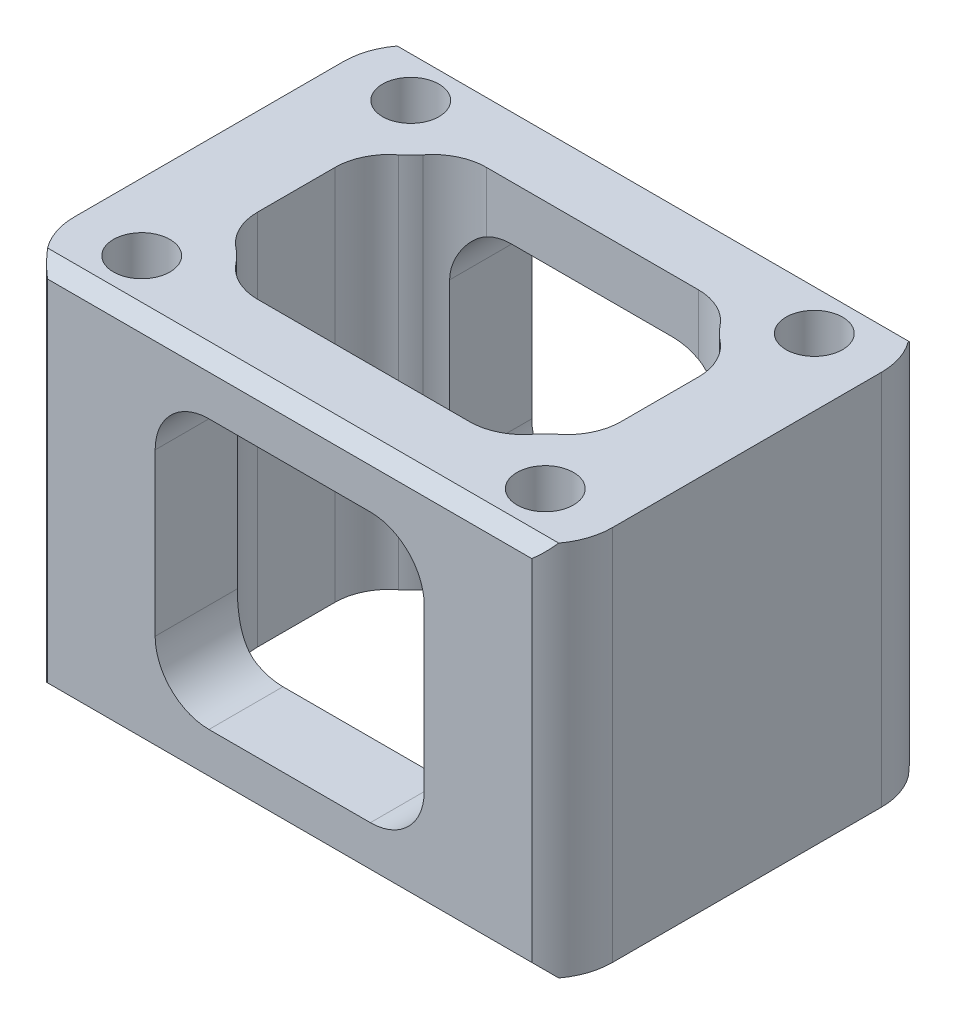
from build123d import *

# Parameters (mm, degrees)
SKETCH_1_W          = 40
SKETCH_1_H          = 28
EXTRUDE_1_DEPTH     = 28
SKETCH_2_R          = 2.1
CUT_EXTRUDE_1_DEPTH = 38.148351242
SKETCH_3_OUTSIDE_W  = 53.256
SKETCH_3_OUTSIDE_H  = 41.256
CUT_EXTRUDE_2_DEPTH = 38.148351242
FILLET_3_R          = 4
SKETCH_6_W          = 20
SKETCH_6_H          = 20
CUT_EXTRUDE_4_DEPTH = 45.362146026
FILLET_4_R          = 4
CHAMFER_1_SIZE      = 1


with BuildPart() as part:
    # 草图1 → 凸台-拉伸1 (new body)
    with BuildSketch(Plane(origin=(0, 0, 0), x_dir=(1, 0, 0), z_dir=(0, 1, 0))):
        Rectangle(SKETCH_1_W, SKETCH_1_H)
    extrude(amount=EXTRUDE_1_DEPTH)

    # 草图2 → 切除-拉伸1 (cut, through all)
    with BuildSketch(Plane(origin=(0, 28, 0), x_dir=(1, 0, 0), z_dir=(0, 1, 0))):
        with Locations(Location((-15, 10, 0), (0, 0, 270))):
            Circle(SKETCH_2_R)
        with Locations(Location((-15, -10, 0), (0, 0, 270))):
            Circle(SKETCH_2_R)
        with Locations(Location((15, -10, 0), (0, 0, 270))):
            Circle(SKETCH_2_R)
        with Locations(Location((15, 10, 0), (0, 0, 270))):
            Circle(SKETCH_2_R)
    extrude(amount=-CUT_EXTRUDE_1_DEPTH, mode=Mode.SUBTRACT)

    # 草图3 outside → 切除-拉伸2 (cut, through all)
    # profile 1 of 2: a face of its own
    with BuildSketch(Plane(origin=(0, 28, 0), x_dir=(1, 0, 0), z_dir=(0, 1, 0))):
        Rectangle(SKETCH_3_OUTSIDE_W, SKETCH_3_OUTSIDE_H)
        with BuildLine():
            Line((20, -10), (20, 10))
            ThreePointArc((20, 10), (17.236067977, 14.472135955), (12, 14))
            Line((12, 14), (-18, 14))
            ThreePointArc((-18, 14), (-19.472135955, 12.236067977), (-20, 10))
            Line((-20, 10), (-20, -10))
            ThreePointArc((-20, -10), (-17.236067977, -14.472135955), (-12, -14))
            Line((-12, -14), (18, -14))
            ThreePointArc((18, -14), (19.472135955, -12.236067977), (20, -10))
        make_face(mode=Mode.SUBTRACT)
    # profile 2 of 2: a face of its own
    with BuildSketch(Plane(origin=(0, 28, 0), x_dir=(1, 0, 0), z_dir=(0, 1, 0))):
        with BuildLine():
            Line((-13.5, -5.230303993), (-13.5, 5.230303993))
            ThreePointArc((-13.5, 5.230303993), (-11.464466094, 6.464466094), (-10.230303993, 8.5))
            Line((-10.230303993, 8.5), (10.230303993, 8.5))
            ThreePointArc((10.230303993, 8.5), (11.464466094, 6.464466094), (13.5, 5.230303993))
            Line((13.5, 5.230303993), (13.5, -5.230303993))
            ThreePointArc((13.5, -5.230303993), (11.464466094, -6.464466094), (10.230303993, -8.5))
            Line((10.230303993, -8.5), (-10.230303993, -8.5))
            ThreePointArc((-10.230303993, -8.5), (-11.464466094, -6.464466094), (-13.5, -5.230303993))
        make_face()
    extrude(amount=-CUT_EXTRUDE_2_DEPTH, mode=Mode.SUBTRACT)

    # 圆角3
    fillet_3_edges = [part.edges().sort_by_distance(p)[0] for p in [
        (-13.5, 14, -5.230303993),
        (-10.230303993, 14, -8.5),
        (10.230303993, 14, -8.5),
        (13.5, 14, -5.230303993),
        (13.5, 14, 5.230303993),
        (10.230303993, 14, 8.5),
        (-10.230303993, 14, 8.5),
        (-13.5, 14, 5.230303993),
    ]]
    fillet(fillet_3_edges, radius=FILLET_3_R)

    # 草图6 → 切除-拉伸4 (cut, through all)
    with BuildSketch(Plane.XY.offset(14)):
        with Locations((0, 14)):
            Rectangle(SKETCH_6_W, SKETCH_6_H)
    extrude(amount=-CUT_EXTRUDE_4_DEPTH, mode=Mode.SUBTRACT)

    # 圆角4
    fillet_4_edges = [part.edges().sort_by_distance(p)[0] for p in [
        (10, 4, -10.944773897),
        (-10, 4, -10.944773897),
        (-10, 24, -10.944773897),
        (10, 24, -10.944773897),
        (10, 4, 10.944773897),
        (-10, 4, 10.944773897),
        (-10, 24, 10.944773897),
        (10, 24, 10.944773897),
    ]]
    fillet(fillet_4_edges, radius=FILLET_4_R)

    # 倒角1
    chamfer_1_edges = [part.edges().sort_by_distance(p)[0] for p in [
        (0, 0, 14),
        (0, 0, -14),
        (0, 28, -14),
        (0, 28, 14),
    ]]
    chamfer(chamfer_1_edges, length=CHAMFER_1_SIZE)


solid = part.part
